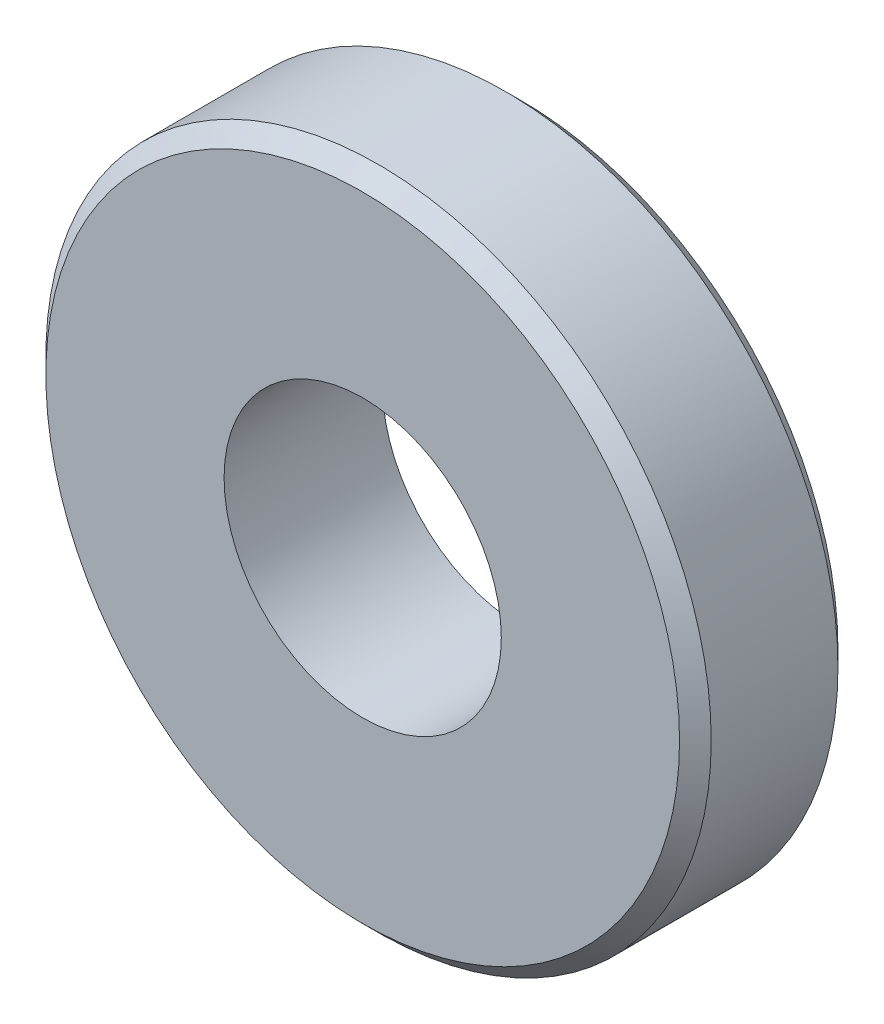
from build123d import *

# Parameters (mm, degrees)
SKETCH1_R           = 210
SKETCH1_R_2         = 87.5
BOSS_EXTRUDE1_DEPTH = 100
CHAMFER1_SIZE       = 10


with BuildPart() as part:
    # Sketch1 → Boss-Extrude1 (new body)
    with BuildSketch(Plane.XY):
        Circle(SKETCH1_R)
        Circle(SKETCH1_R_2, mode=Mode.SUBTRACT)
    extrude(amount=BOSS_EXTRUDE1_DEPTH)

    # Chamfer1
    chamfer1_edges = [part.edges().sort_by_distance(p)[0] for p in [
        (-210, 0, 0),
        (-210, 0, 100),
    ]]
    chamfer(chamfer1_edges, length=CHAMFER1_SIZE)


solid = part.part
